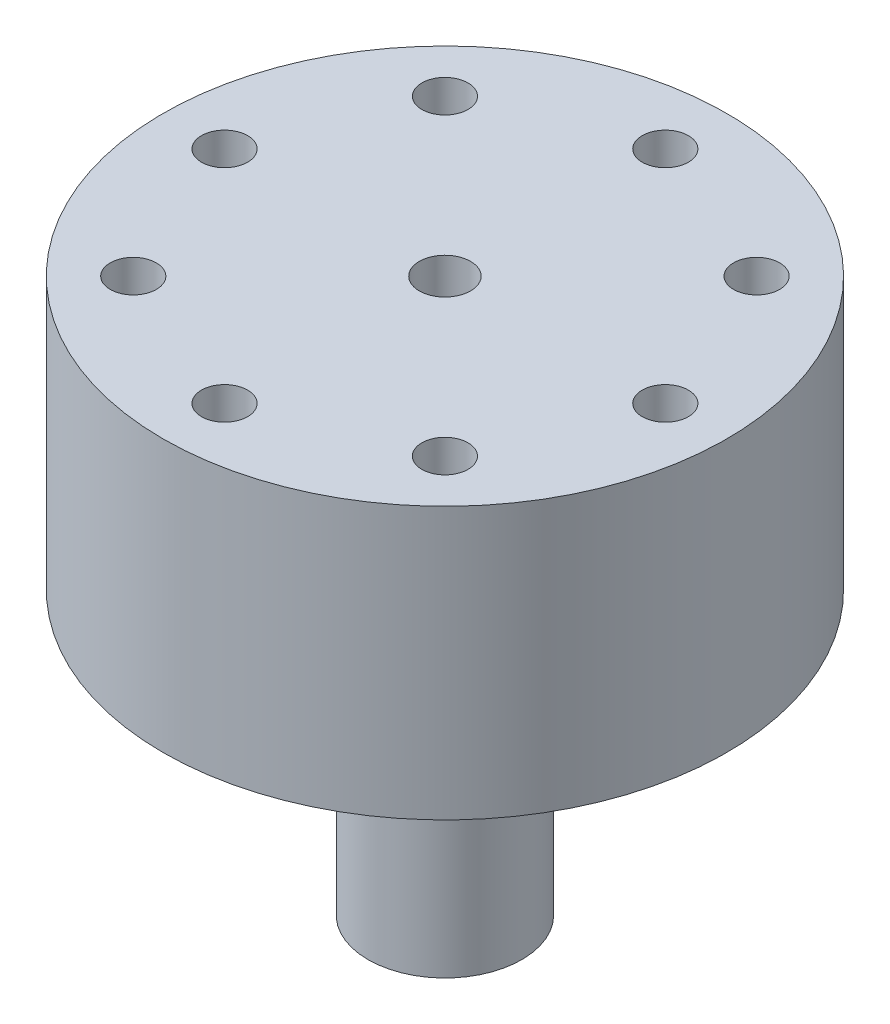
from build123d import *

# Parameters (mm, degrees)
SKETCH_2_R          = 7.5
CUT_EXTRUDE_1_DEPTH = 2
CUT_EXTRUDE_2_REACH = 95.011
SKETCH_5_R          = 4.5
SKETCH_7_R          = 30.721623485
EXTRUDE_1_DEPTH     = 41
SKETCH_8_R          = 17.5
EXTRUDE_2_DEPTH     = 10
SKETCH_9_R          = 15
EXTRUDE_3_DEPTH     = 45
SKETCH_10_R         = 15
SKETCH_10_R_2       = 13
CUT_EXTRUDE_3_DEPTH = 2


with BuildPart() as part:
    # 草图1 → 旋转1 (revolve)
    with BuildSketch(Plane.XY, mode=Mode.PRIVATE) as revolve_1_sk:
        with BuildLine():
            Line((5, 13.223493336), (5, 0.265127902))
            ThreePointArc((5, 0.265127902), (24.788681465, -14.86973249), (24.233241632, -39.776506664))
            Line((24.233241632, -39.776506664), (55, -39.776506664))
            Line((55, -39.776506664), (55, 13.223493336))
            Line((55, 13.223493336), (5, 13.223493336))
        make_face()
    revolve(revolve_1_sk.sketch.rotate(Axis((0, 13.888286008, 0), (0, -1, 0)), 90), axis=Axis((0, 13.888286008, 0), (0, -1, 0)))

    # 草图2 → 切除-拉伸1 (cut)
    with BuildSketch(Plane.XZ.offset(39.776506664)):
        with Locations(Location((43, 0, 0), (0, 0, 270))):
            Circle(SKETCH_2_R)
        with Locations(Location((30.405591591, -30.405591591, 0), (0, 0, 270))):
            Circle(SKETCH_2_R)
        with Locations(Location((0, -43, 0), (0, 0, 270))):
            Circle(SKETCH_2_R)
        with Locations(Location((-30.405591591, -30.405591591, 0), (0, 0, 270))):
            Circle(SKETCH_2_R)
        with Locations(Location((-43, 0, 0), (0, 0, 270))):
            Circle(SKETCH_2_R)
        with Locations(Location((-30.405591591, 30.405591591, 0), (0, 0, 270))):
            Circle(SKETCH_2_R)
        with Locations(Location((0, 43, 0), (0, 0, 270))):
            Circle(SKETCH_2_R)
        with Locations(Location((30.405591591, 30.405591591, 0), (0, 0, 270))):
            Circle(SKETCH_2_R)
    extrude(amount=-CUT_EXTRUDE_1_DEPTH, mode=Mode.SUBTRACT)

    # 草图5 → 切除-拉伸2 (cut, up to next)
    with BuildSketch(Plane.XZ.offset(37.776506664), mode=Mode.PRIVATE) as cut_extrude_2_sk1:
        with Locations(Location((0, 43, 0), (0, 0, 270))):
            Circle(SKETCH_5_R)
    cut_extrude_2_tool1 = extrude(cut_extrude_2_sk1.sketch, amount=-CUT_EXTRUDE_2_REACH, mode=Mode.PRIVATE) & part.part
    # 草图5 → 切除-拉伸2 (cut, up to next)
    with BuildSketch(Plane.XZ.offset(37.776506664), mode=Mode.PRIVATE) as cut_extrude_2_sk2:
        with Locations(Location((30.405591591, 30.405591591, 0), (0, 0, 270))):
            Circle(SKETCH_5_R)
    cut_extrude_2_tool2 = extrude(cut_extrude_2_sk2.sketch, amount=-CUT_EXTRUDE_2_REACH, mode=Mode.PRIVATE) & part.part
    # 草图5 → 切除-拉伸2 (cut, up to next)
    with BuildSketch(Plane.XZ.offset(37.776506664), mode=Mode.PRIVATE) as cut_extrude_2_sk3:
        with Locations(Location((43, 0, 0), (0, 0, 270))):
            Circle(SKETCH_5_R)
    cut_extrude_2_tool3 = extrude(cut_extrude_2_sk3.sketch, amount=-CUT_EXTRUDE_2_REACH, mode=Mode.PRIVATE) & part.part
    # 草图5 → 切除-拉伸2 (cut, up to next)
    with BuildSketch(Plane.XZ.offset(37.776506664), mode=Mode.PRIVATE) as cut_extrude_2_sk4:
        with Locations(Location((30.405591591, -30.405591591, 0), (0, 0, 270))):
            Circle(SKETCH_5_R)
    cut_extrude_2_tool4 = extrude(cut_extrude_2_sk4.sketch, amount=-CUT_EXTRUDE_2_REACH, mode=Mode.PRIVATE) & part.part
    # 草图5 → 切除-拉伸2 (cut, up to next)
    with BuildSketch(Plane.XZ.offset(37.776506664), mode=Mode.PRIVATE) as cut_extrude_2_sk5:
        with Locations(Location((0, -43, 0), (0, 0, 270))):
            Circle(SKETCH_5_R)
    cut_extrude_2_tool5 = extrude(cut_extrude_2_sk5.sketch, amount=-CUT_EXTRUDE_2_REACH, mode=Mode.PRIVATE) & part.part
    # 草图5 → 切除-拉伸2 (cut, up to next)
    with BuildSketch(Plane.XZ.offset(37.776506664), mode=Mode.PRIVATE) as cut_extrude_2_sk6:
        with Locations(Location((-30.405591591, -30.405591591, 0), (0, 0, 270))):
            Circle(SKETCH_5_R)
    cut_extrude_2_tool6 = extrude(cut_extrude_2_sk6.sketch, amount=-CUT_EXTRUDE_2_REACH, mode=Mode.PRIVATE) & part.part
    # 草图5 → 切除-拉伸2 (cut, up to next)
    with BuildSketch(Plane.XZ.offset(37.776506664), mode=Mode.PRIVATE) as cut_extrude_2_sk7:
        with Locations(Location((-43, 0, 0), (0, 0, 270))):
            Circle(SKETCH_5_R)
    cut_extrude_2_tool7 = extrude(cut_extrude_2_sk7.sketch, amount=-CUT_EXTRUDE_2_REACH, mode=Mode.PRIVATE) & part.part
    # 草图5 → 切除-拉伸2 (cut, up to next)
    with BuildSketch(Plane.XZ.offset(37.776506664), mode=Mode.PRIVATE) as cut_extrude_2_sk8:
        with Locations(Location((-30.405591591, 30.405591591, 0), (0, 0, 270))):
            Circle(SKETCH_5_R)
    cut_extrude_2_tool8 = extrude(cut_extrude_2_sk8.sketch, amount=-CUT_EXTRUDE_2_REACH, mode=Mode.PRIVATE) & part.part
    add(cut_extrude_2_tool1.solids().sort_by_distance((0, -37.776507, 43))[0], mode=Mode.SUBTRACT)
    add(cut_extrude_2_tool2.solids().sort_by_distance((30.405592, -37.776507, 30.405592))[0], mode=Mode.SUBTRACT)
    add(cut_extrude_2_tool3.solids().sort_by_distance((43, -37.776507, 0))[0], mode=Mode.SUBTRACT)
    add(cut_extrude_2_tool4.solids().sort_by_distance((30.405592, -37.776507, -30.405592))[0], mode=Mode.SUBTRACT)
    add(cut_extrude_2_tool5.solids().sort_by_distance((0, -37.776507, -43))[0], mode=Mode.SUBTRACT)
    add(cut_extrude_2_tool6.solids().sort_by_distance((-30.405592, -37.776507, -30.405592))[0], mode=Mode.SUBTRACT)
    add(cut_extrude_2_tool7.solids().sort_by_distance((-43, -37.776507, 0))[0], mode=Mode.SUBTRACT)
    add(cut_extrude_2_tool8.solids().sort_by_distance((-30.405592, -37.776507, 30.405592))[0], mode=Mode.SUBTRACT)

    # 草图7 → 凸台-拉伸1 (add)
    with BuildSketch(Plane.XZ.offset(39.776506664)):
        Circle(SKETCH_7_R)
    extrude(amount=-EXTRUDE_1_DEPTH)

    # 草图8 → 凸台-拉伸2 (add)
    with BuildSketch(Plane.XZ.offset(39.776506664)):
        with Locations(Location((0, 0, 0), (0, 0, 270))):
            Circle(SKETCH_8_R)
    extrude(amount=EXTRUDE_2_DEPTH)

    # 草图9 → 凸台-拉伸3 (add)
    with BuildSketch(Plane.XZ.offset(49.776506664)):
        with Locations(Location((0, 0, 0), (0, 0, 90))):
            Circle(SKETCH_9_R)
    extrude(amount=EXTRUDE_3_DEPTH)

    # 草图10 → 切除-拉伸3 (cut)
    with BuildSketch(Plane.XZ.offset(49.776506664)):
        with Locations(Location((0, 0, 0), (0, 0, 90))):
            Circle(SKETCH_10_R)
        with Locations(Location((0, 0, 0), (0, 0, 270))):
            Circle(SKETCH_10_R_2, mode=Mode.SUBTRACT)
    extrude(amount=CUT_EXTRUDE_3_DEPTH, mode=Mode.SUBTRACT)


solid = part.part
